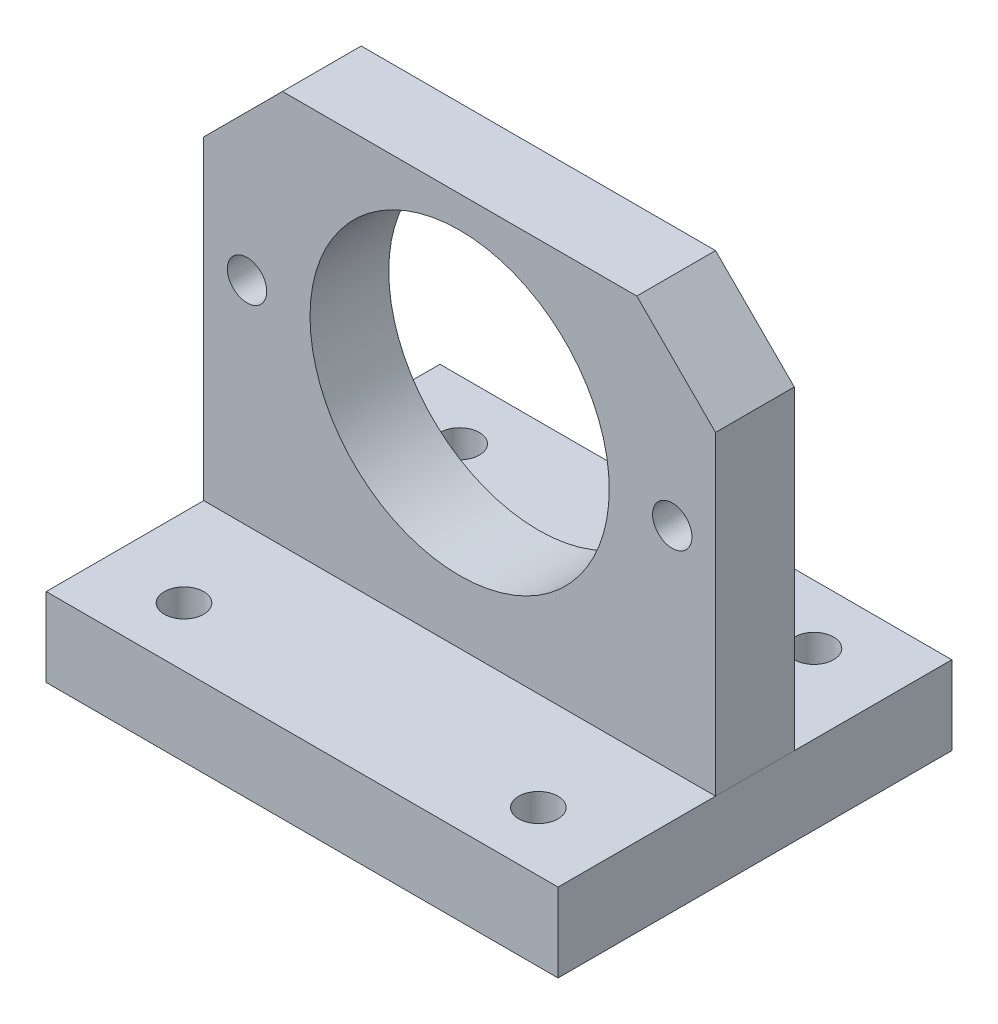
from build123d import *

# Parameters (mm, degrees)
SKETCH1_W                  = 65
SKETCH1_H                  = 50
BOSS_EXTRUDE1_DEPTH        = 10
SKETCH2_W                  = 65
SKETCH2_H                  = 10
BOSS_EXTRUDE2_DEPTH        = 50
SKETCH3_R                  = 19
CUT_EXTRUDE1_DEPTH         = 10
CHAMFER1_SIZE              = 10
SKETCH5_W                  = 2.5
SKETCH5_H                  = 10
M6_TAPPED_HOLE2_AT_2_COUNT = 2
M6_TAPPED_HOLE2_AT_2_PITCH = 57.008771255
M6_TAPPED_HOLE2_AT_3_COUNT = 2
M6_TAPPED_HOLE2_AT_3_PITCH = 45
M6_TAPPED_HOLE2_AT_4_COUNT = 2
M6_TAPPED_HOLE2_AT_4_PITCH = 35
SKETCH7_W                  = 2.5
SKETCH7_H                  = 10
M6_TAPPED_HOLE1_AT_2_COUNT = 2
M6_TAPPED_HOLE1_AT_2_PITCH = 54


with BuildPart() as part:
    # Sketch1 → Boss-Extrude1 (new body)
    with BuildSketch(Plane(origin=(0, 0, 0), x_dir=(1, 0, 0), z_dir=(0, 1, 0))):
        Rectangle(SKETCH1_W, SKETCH1_H)
    extrude(amount=BOSS_EXTRUDE1_DEPTH)

    # Sketch5 → M6 Tapped Hole2 (revolve, cut)
    with BuildSketch(Plane(origin=(22.5, 10, 17.5), x_dir=(0, 0, 1), z_dir=(1, 0, 0))):
        with Locations((1.25, 5)):
            Rectangle(SKETCH5_W, SKETCH5_H)
    m6_tapped_hole2 = revolve(axis=Axis((22.5, 16.35, 17.5), (0, -1, 0)), mode=Mode.SUBTRACT)

    # M6 Tapped Hole2 at 2: M6 Tapped Hole2 ×2
    with Locations(*[Vector(-0.7893522173763263, 0, -0.6139406135149205) * (i * M6_TAPPED_HOLE2_AT_2_PITCH) for i in range(1, M6_TAPPED_HOLE2_AT_2_COUNT)]):
        add(m6_tapped_hole2, mode=Mode.SUBTRACT)

    # M6 Tapped Hole2 at 3: M6 Tapped Hole2 ×2
    with Locations(*[(-i * M6_TAPPED_HOLE2_AT_3_PITCH, 0, 0) for i in range(1, M6_TAPPED_HOLE2_AT_3_COUNT)]):
        add(m6_tapped_hole2, mode=Mode.SUBTRACT)

    # M6 Tapped Hole2 at 4: M6 Tapped Hole2 ×2
    with Locations(*[(0, 0, -i * M6_TAPPED_HOLE2_AT_4_PITCH) for i in range(1, M6_TAPPED_HOLE2_AT_4_COUNT)]):
        add(m6_tapped_hole2, mode=Mode.SUBTRACT)


with BuildPart() as body_2:
    # Sketch2 → Boss-Extrude2 (new body)
    with BuildSketch(Plane(origin=(0, 10, 0), x_dir=(1, 0, 0), z_dir=(0, 1, 0))):
        Rectangle(SKETCH2_W, SKETCH2_H)
    extrude(amount=BOSS_EXTRUDE2_DEPTH)

    # Sketch3 → Cut-Extrude1 (cut)
    with BuildSketch(Plane.XY.offset(5)):
        with Locations((0, 37)):
            Circle(SKETCH3_R)
    extrude(amount=-CUT_EXTRUDE1_DEPTH, mode=Mode.SUBTRACT)

    # Chamfer1
    chamfer1_edges = [body_2.edges().sort_by_distance(p)[0] for p in [
        (-32.5, 60, 0),
        (32.5, 60, 0),
    ]]
    chamfer(chamfer1_edges, length=CHAMFER1_SIZE)

    # Sketch7 → M6 Tapped Hole1 (revolve, cut)
    with BuildSketch(Plane(origin=(-27, 37, 5), x_dir=(0, -1, 0), z_dir=(1, 0, 0))):
        with Locations((1.25, 5)):
            Rectangle(SKETCH7_W, SKETCH7_H)
    m6_tapped_hole1 = revolve(axis=Axis((-27, 37, 11.35), (0, 0, -1)), mode=Mode.SUBTRACT)

    # M6 Tapped Hole1 at 2: M6 Tapped Hole1 ×2
    with Locations(*[(i * M6_TAPPED_HOLE1_AT_2_PITCH, 0, 0) for i in range(1, M6_TAPPED_HOLE1_AT_2_COUNT)]):
        add(m6_tapped_hole1, mode=Mode.SUBTRACT)


solid = Compound([part.part, body_2.part])
